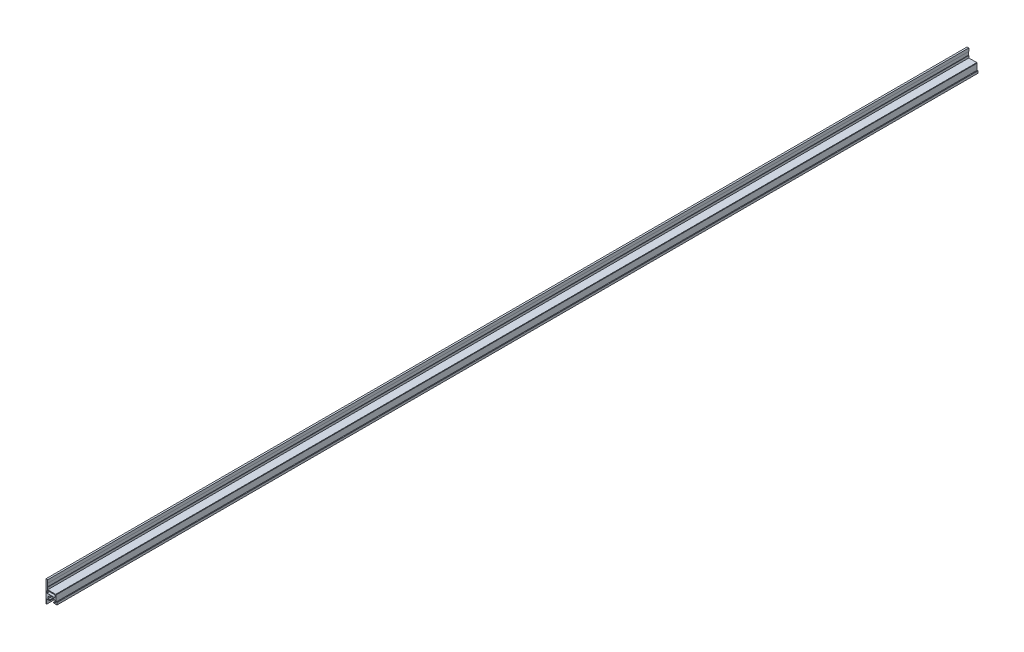
from build123d import *

# Parameters (mm, degrees)
SKETCH_2_W      = 19
SKETCH_2_H      = 5.6
EXTRUDE_1_DEPTH = 1058


with BuildPart() as part:
    # 草图2 → 凸台-拉伸1 (new, symmetric)
    with BuildSketch(Plane.XY):
        with BuildLine():
            Line((1.5, 10), (4, 10))
            Line((4, 10), (4, 10.5))
            Line((4, 10.5), (8.9, 10.5))
            Line((8.9, 10.5), (8.9, 12.2))
            ThreePointArc((8.9, 12.2), (8.812132034, 12.412132034), (8.6, 12.5))
            Line((8.6, 12.5), (5.05, 12.5))
            ThreePointArc((5.05, 12.5), (4.837867966, 12.587867966), (4.75, 12.8))
            Line((4.75, 12.8), (4.75, 16.152943725))
            ThreePointArc((4.75, 16.152943725), (4.77283614, 16.267748755), (4.837867966, 16.36507576))
            Line((4.837867966, 16.36507576), (8.78492424, 20.312132034))
            ThreePointArc((8.78492424, 20.312132034), (8.882251245, 20.37716386), (8.997056275, 20.4))
            Line((8.997056275, 20.4), (17.002943725, 20.4))
            ThreePointArc((17.002943725, 20.4), (17.117748755, 20.37716386), (17.21507576, 20.312132034))
            Line((17.21507576, 20.312132034), (21.162132034, 16.36507576))
            ThreePointArc((21.162132034, 16.36507576), (21.22716386, 16.267748755), (21.25, 16.152943725))
            Line((21.25, 16.152943725), (21.25, 12.8))
            ThreePointArc((21.25, 12.8), (21.162132034, 12.587867966), (20.95, 12.5))
            Line((20.95, 12.5), (17.4, 12.5))
            ThreePointArc((17.4, 12.5), (17.187867966, 12.412132034), (17.1, 12.2))
            Line((17.1, 12.2), (17.1, 10.5))
            Line((17.1, 10.5), (22, 10.5))
            Line((22, 10.5), (22, 10))
            Line((22, 10), (25, 10))
            Line((25, 10), (25, 15))
            Line((25, 15), (23, 15))
            Line((23, 15), (23, 29.24572809))
            Line((23, 29.24572809), (22.25, 29.99572809))
            Line((22.25, 29.99572809), (4, 30))
            Line((4, 30), (4, 34.998393128))
            Line((4, 34.998393128), (3, 34.998393128))
            Line((3, 34.998393128), (3, 43))
            Line((3, 43), (4, 43))
            Line((4, 43), (4, 50))
            Line((4, 50), (0, 50))
            Line((0, 50), (0, 0))
            Line((0, 0), (1.5, 0))
            Line((1.5, 0), (1.5, 10))
        make_face()
        with Locations((11.5, 25.2)):
            Rectangle(SKETCH_2_W, SKETCH_2_H, mode=Mode.SUBTRACT)
    extrude(amount=EXTRUDE_1_DEPTH, both=True)


solid = part.part
